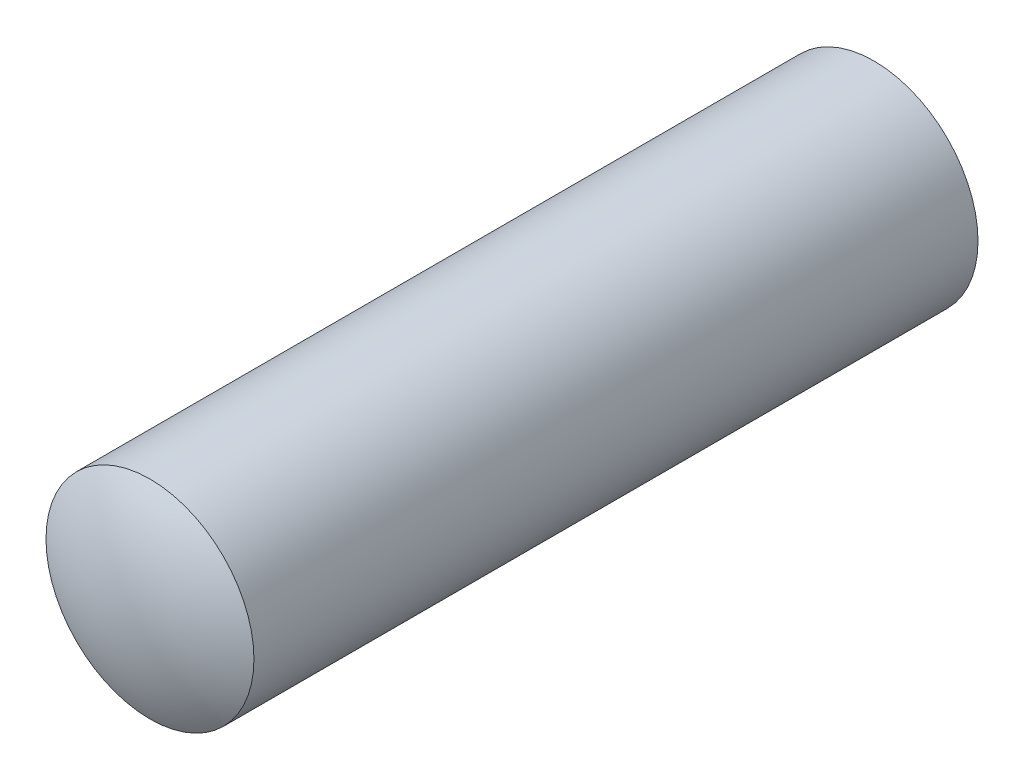
from build123d import *


with BuildPart() as part:
    # Logo3_bib1 → Revolve1 (revolve)
    with BuildSketch(Plane(origin=(0, 0, 0), x_dir=(-1, 0, 0), z_dir=(0, -1, 0))):
        with BuildLine():
            Line((0, 8), (0, -7))
            ThreePointArc((0, -7), (1.03527618, -6.863703305), (2, -6.464101615))
            Line((2, -6.464101615), (2, 7.464101615))
            ThreePointArc((2, 7.464101615), (1.03527618, 7.863703305), (0, 8))
        make_face()
    revolve(axis=Axis((0, 0, -47.537203702), (0, 0, 1)))


solid = part.part
